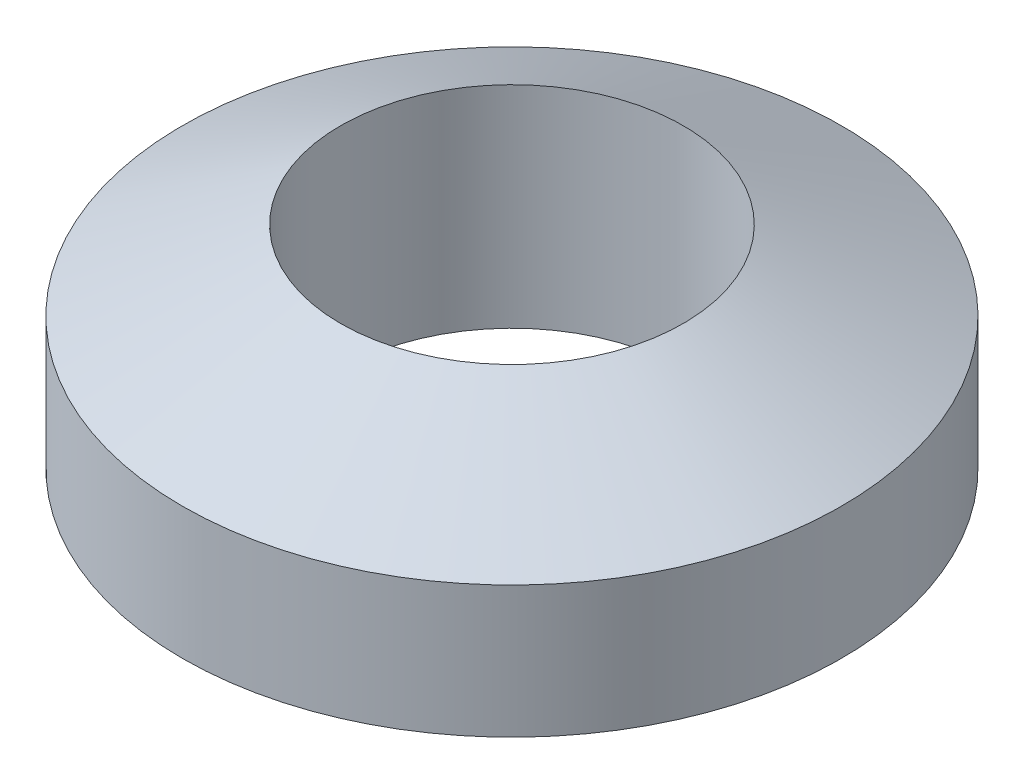
from build123d import *

# Parameters (mm, degrees)
SKETCH_2_R          = 5
CUT_EXTRUDE_1_DEPTH = 30


with BuildPart() as part:
    # 草图1 → 旋转1 (revolve)
    with BuildSketch(Plane.XY, mode=Mode.PRIVATE) as revolve_1_sk:
        Polygon((65, -53.991935484), (65, 26.008064516), (125, -3.991935484), (125, -53.991935484), align=None)
    revolve(revolve_1_sk.sketch.rotate(Axis((0, 116.89516129, 0), (0, -1, 0)), 90), axis=Axis((0, 116.89516129, 0), (0, -1, 0)))

    # 草图2 → 切除-拉伸1 (cut)
    with BuildSketch(Plane.XZ.offset(53.991935484)):
        with Locations(Location((90, 0, 0), (0, 0, 270))):
            Circle(SKETCH_2_R)
        with Locations(Location((63.639610307, -63.639610307, 0), (0, 0, 270))):
            Circle(SKETCH_2_R)
        with Locations(Location((0, -90, 0), (0, 0, 270))):
            Circle(SKETCH_2_R)
        with Locations(Location((-63.639610307, -63.639610307, 0), (0, 0, 270))):
            Circle(SKETCH_2_R)
        with Locations(Location((-90, 0, 0), (0, 0, 270))):
            Circle(SKETCH_2_R)
        with Locations(Location((-63.639610307, 63.639610307, 0), (0, 0, 270))):
            Circle(SKETCH_2_R)
        with Locations(Location((0, 90, 0), (0, 0, 270))):
            Circle(SKETCH_2_R)
        with Locations(Location((63.639610307, 63.639610307, 0), (0, 0, 270))):
            Circle(SKETCH_2_R)
    extrude(amount=-CUT_EXTRUDE_1_DEPTH, mode=Mode.SUBTRACT)


solid = part.part
